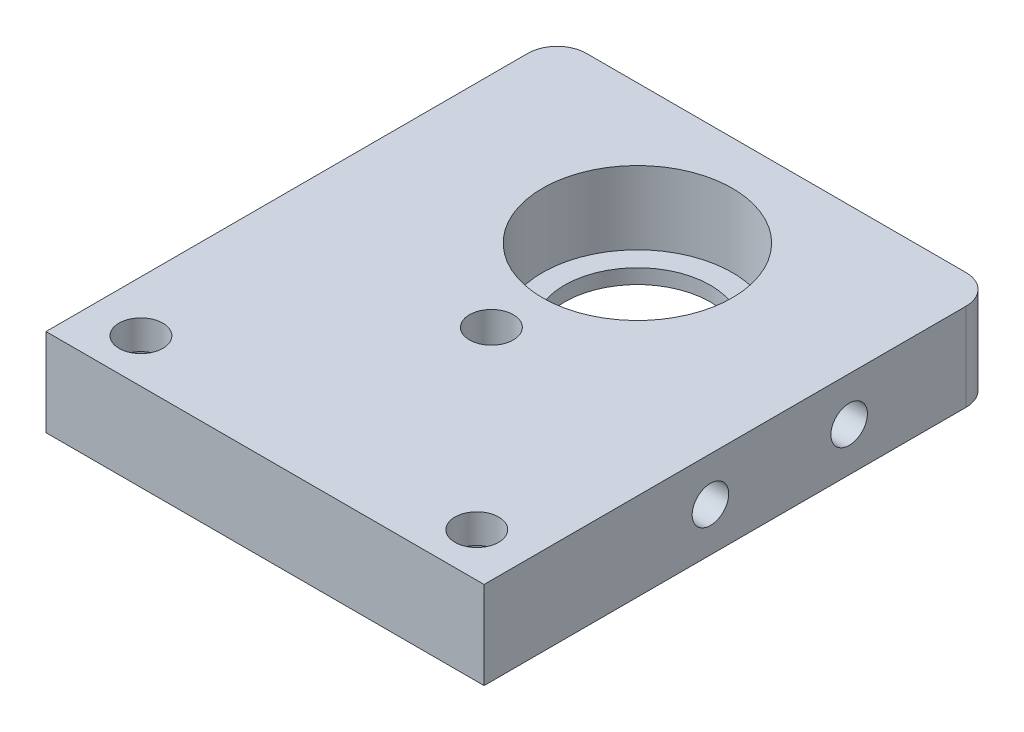
from build123d import *

# Parameters (mm, degrees)
SKETCH1_R             = 5
SKETCH1_R_2           = 1.5
BOSS_EXTRUDE1_DEPTH   = 6
SKETCH3_R             = 6.5
CUT_EXTRUDE1_DEPTH    = 5
SKETCH4_R             = 1.5
CUT_EXTRUDE2_DEPTH    = 24.817010728
SKETCH5_R             = 2.5
CUT_EXTRUDE3_DEPTH    = 4
SKETCH8_R             = 1
CUT_EXTRUDE6_DEPTH    = 2
M3_TAPPED_HOLE1_D     = 2.5
M3_TAPPED_HOLE1_DEPTH = 7.5
M3_TAPPED_HOLE1_TIP   = 0.751075774


with BuildPart() as part:
    # Sketch1 → Boss-Extrude1 (new body)
    with BuildSketch(Plane(origin=(0, 0, 0), x_dir=(1, 0, 0), z_dir=(0, 1, 0))):
        with BuildLine():
            Line((-13, 17.5), (13, 17.5))
            ThreePointArc((13, 17.5), (14.414213562, 16.914213562), (15, 15.5))
            Line((15, 15.5), (15, -17.5))
            Line((15, -17.5), (-15, -17.5))
            Line((-15, -17.5), (-15, 15.5))
            ThreePointArc((-15, 15.5), (-14.414213562, 16.914213562), (-13, 17.5))
        make_face()
        with Locations(Location((0, 8, 0), (0, 0, 270))):
            Circle(SKETCH1_R, mode=Mode.SUBTRACT)
        with Locations(Location((0, -2, 0), (0, 0, 270))):
            Circle(SKETCH1_R_2, mode=Mode.SUBTRACT)
    extrude(amount=BOSS_EXTRUDE1_DEPTH)

    # Sketch3 → Cut-Extrude1 (cut)
    with BuildSketch(Plane(origin=(0, 6, 0), x_dir=(1, 0, 0), z_dir=(0, 1, 0))):
        with Locations(Location((0, 8, 0), (0, 0, 270))):
            Circle(SKETCH3_R)
    extrude(amount=-CUT_EXTRUDE1_DEPTH, mode=Mode.SUBTRACT)

    # Sketch4 → Cut-Extrude2 (cut, through all)
    with BuildSketch(Plane(origin=(0, 6, 0), x_dir=(1, 0, 0), z_dir=(0, 1, 0))):
        with Locations(Location((-11.5, -14.5, 0), (0, 0, 270))):
            Circle(SKETCH4_R)
        with Locations(Location((11.5, -14.5, 0), (0, 0, 270))):
            Circle(SKETCH4_R)
    extrude(amount=-CUT_EXTRUDE2_DEPTH, mode=Mode.SUBTRACT)

    # Sketch5 → Cut-Extrude3 (cut)
    with BuildSketch(Plane.XZ):
        with Locations(Location((11.5, 14.5, 0), (0, 0, 270))):
            Circle(SKETCH5_R)
        with Locations(Location((-11.5, 14.5, 0), (0, 0, 270))):
            Circle(SKETCH5_R)
    extrude(amount=-CUT_EXTRUDE3_DEPTH, mode=Mode.SUBTRACT)

    # Sketch8 → Cut-Extrude6 (cut)
    with BuildSketch(Plane(origin=(15, 0, 0), x_dir=(0, 0, -1), z_dir=(1, 0, 0))):
        with Locations((-2, 3)):
            Circle(SKETCH8_R)
        with Locations((7.5, 3)):
            Circle(SKETCH8_R)
    extrude(amount=-CUT_EXTRUDE6_DEPTH, mode=Mode.SUBTRACT)

    # M3 Tapped Hole1
    with Locations(Plane(origin=(15, 0, 0), x_dir=(0, 0, -1), z_dir=(1, 0, 0))):
        with Locations((-2, 3), (7.5, 3)):
            Hole(M3_TAPPED_HOLE1_D / 2, depth=M3_TAPPED_HOLE1_DEPTH)
            with Locations((0, 0, -(M3_TAPPED_HOLE1_DEPTH + M3_TAPPED_HOLE1_TIP / 2))):  # 118° drill point
                Cone(0, M3_TAPPED_HOLE1_D / 2, M3_TAPPED_HOLE1_TIP, mode=Mode.SUBTRACT)


solid = part.part
